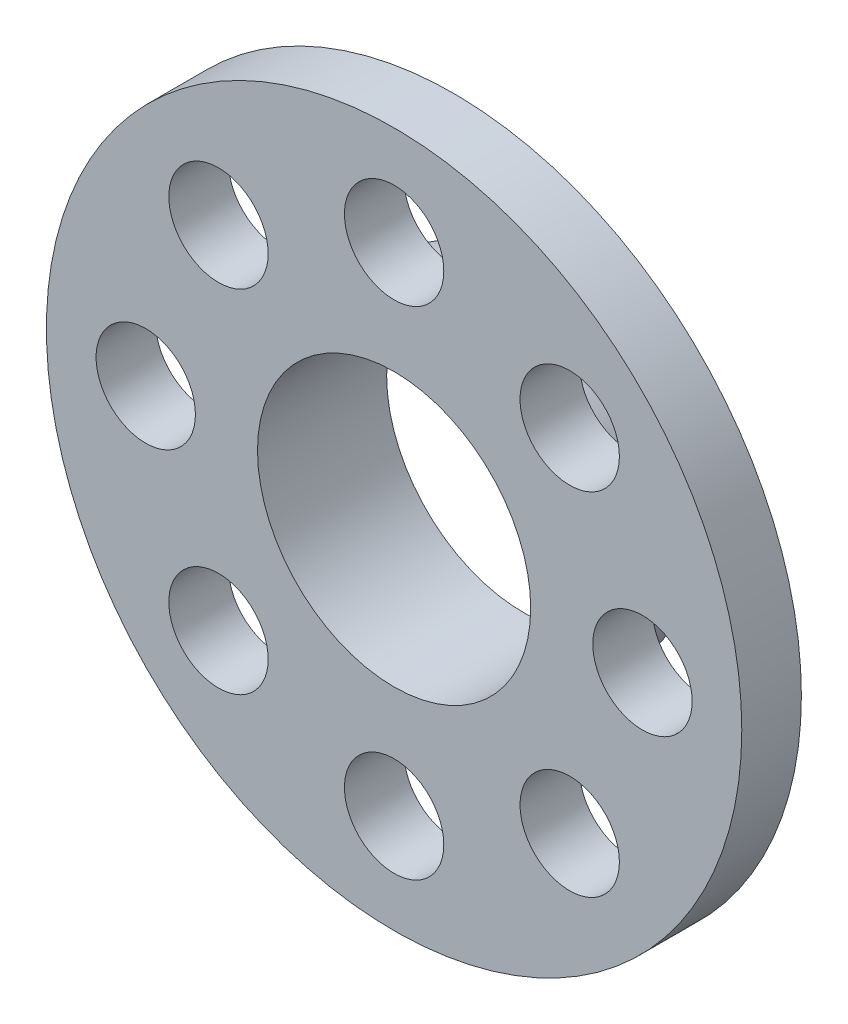
from build123d import *
from build123d.topology import SkipClean

# Parameters (mm, degrees)
SKETCH2_R           = 70
SKETCH2_R_2         = 27.5
BOSS_EXTRUDE1_DEPTH = 12
SKETCH3_R           = 10
CUT_EXTRUDE1_DEPTH  = 100.719606899
CIRPATTERN1_COUNT   = 8
BOSS_EXTRUDE2_START = 14
SKETCH4_R           = 33.5
SKETCH4_R_2         = 27.5
BOSS_EXTRUDE2_DEPTH = 14


with BuildPart() as part:
    # Sketch2 → Boss-Extrude1 (new body)
    with BuildSketch(Plane.XY):
        Circle(SKETCH2_R)
        Circle(SKETCH2_R_2, mode=Mode.SUBTRACT)
    extrude(amount=BOSS_EXTRUDE1_DEPTH)

    # Sketch3 → Cut-Extrude1 (cut, symmetric)
    with BuildSketch(Plane.XY.offset(12)):
        with Locations((0, -50)):
            Circle(SKETCH3_R)
    cut_extrude1 = extrude(amount=CUT_EXTRUDE1_DEPTH, both=True, mode=Mode.SUBTRACT)

    # CirPattern1: Cut-Extrude1 ×8 about axis
    cirpattern1_axis = Axis((0, 0, 0), (0, 0, 1))
    for i in range(1, CIRPATTERN1_COUNT):
        add(cut_extrude1.rotate(cirpattern1_axis, i * 360 / CIRPATTERN1_COUNT), mode=Mode.SUBTRACT)

    # Sketch4 → Boss-Extrude2 (add)
    with SkipClean():  # the faces are left unmerged after this step: merging them gives an invalid solid
        with BuildSketch(Plane(origin=(0, 0, 0), x_dir=(-1, 0, 0), z_dir=(0, 0, -1)).offset(BOSS_EXTRUDE2_START)):
            with Locations(Location((0, 0, 0), (0, 0, 180))):
                Circle(SKETCH4_R)
            Circle(SKETCH4_R_2, mode=Mode.SUBTRACT)
        extrude(amount=-BOSS_EXTRUDE2_DEPTH)


solid = part.part
